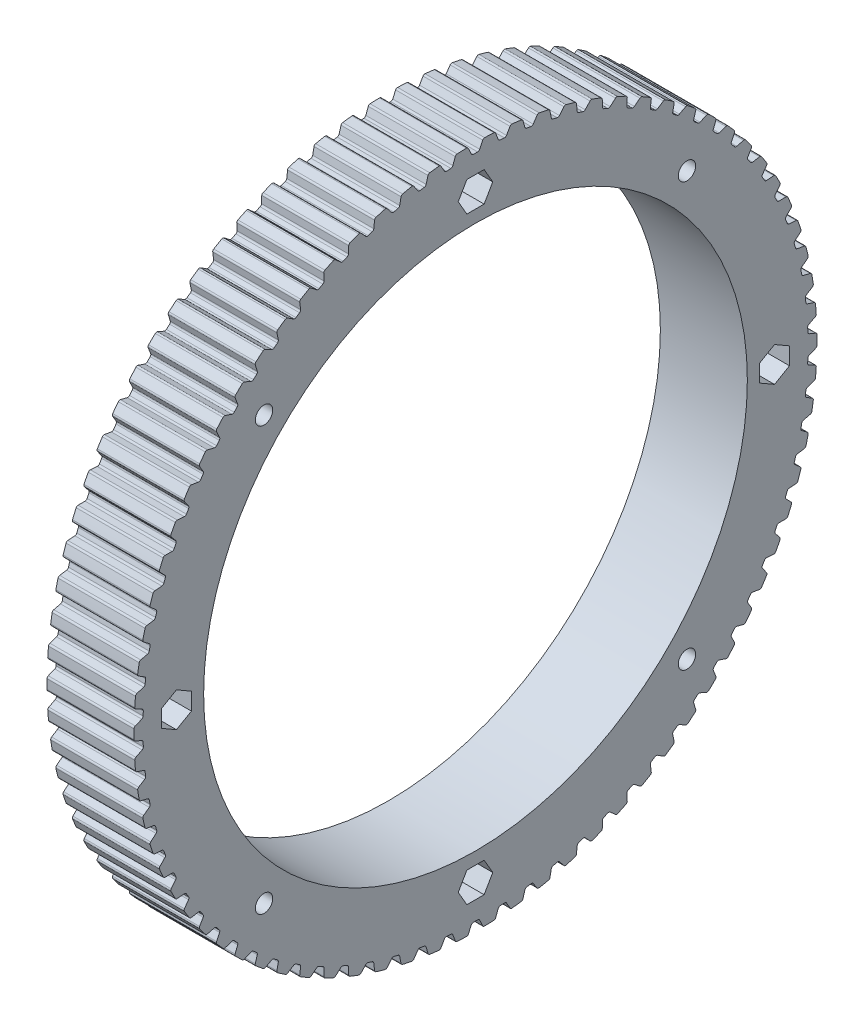
from build123d import *

# Parameters (mm, degrees)
CHAMFER_1_SIZE           = 1
SKETCH_4_W               = 8
SKETCH_4_H               = 3.299999952
CUT_EXTRUDE_1_DEPTH      = 91.633566861
CUT_EXTRUDE_2_REACH      = 92.634
PATTERN_CIRCULAR_3_COUNT = 78
CUT_EXTRUDE_4_DEPTH      = 91.242238534
CUT_EXTRUDE_4_DEPTH_BACK = 91.242238534
SKETCH_7_R               = 50
SKETCH_7_R_2             = 1.6
CUT_EXTRUDE_5_DEPTH      = 5
CUT_EXTRUDE_6_DEPTH      = 5


with BuildPart() as part:
    # 草图1 → 旋转1 (revolve)
    with BuildSketch(Plane.XY, mode=Mode.PRIVATE) as revolve_1_sk:
        Polygon((0, 11.5922), (0, 62.811), (16, 62.811), (16, 23.1844), (18, 23.1844), (18, 11.5922), align=None)
    revolve(revolve_1_sk.sketch.rotate(Axis((0, 0, 0), (1, 0, 0)), 90), axis=Axis((0, 0, 0), (1, 0, 0)))

    # 倒角1
    chamfer_1_edges = [part.edges().sort_by_distance(p)[0] for p in [
        (0, 0, -11.5922),
        (18, 0, -11.5922),
    ]]
    chamfer(chamfer_1_edges, length=CHAMFER_1_SIZE)

    # 草图4 → 切除-拉伸1 (cut, through all)
    with BuildSketch(Plane.ZY):
        with Locations((0, 12.530216005)):
            Rectangle(SKETCH_4_W, SKETCH_4_H)
    extrude(amount=-CUT_EXTRUDE_1_DEPTH, mode=Mode.SUBTRACT)

    # 草图6 → 切除-拉伸2 (cut, up to next)
    with BuildSketch(Plane(origin=(0, 0, 0), x_dir=(0, 0, -1), z_dir=(1, 0, 0)), mode=Mode.PRIVATE) as cut_extrude_2_sk1:
        with BuildLine():
            Line((1.318430055, 62.569446614), (0.771442548, 61.396428119))
            ThreePointArc((0.771442548, 61.396428119), (0.619025206, 61.223197616), (0.39719372, 61.159710252))
            ThreePointArc((0.39719372, 61.159710252), (0, 61.161), (-0.39719372, 61.159710252))
            ThreePointArc((-0.39719372, 61.159710252), (-0.619025206, 61.223197616), (-0.771442548, 61.396428119))
            Line((-0.771442548, 61.396428119), (-1.318430055, 62.569446614))
            ThreePointArc((-1.318430055, 62.569446614), (-1.462939702, 62.732031287), (-1.672948176, 62.788716864))
            ThreePointArc((-1.672948176, 62.788716864), (-1.862873117, 62.783369014), (-2.052781012, 62.777446676))
            Line((-2.052781012, 62.777446676), (-2.66825474, 64.097334344))
            ThreePointArc((-2.66825474, 64.097334344), (0, 64.152847586), (2.66825474, 64.097334344))
            Line((2.66825474, 64.097334344), (2.052781012, 62.777446676))
            ThreePointArc((2.052781012, 62.777446676), (1.862873117, 62.783369014), (1.672948176, 62.788716864))
            ThreePointArc((1.672948176, 62.788716864), (1.462939702, 62.732031287), (1.318430055, 62.569446614))
        make_face()
    cut_extrude_2_tool1 = extrude(cut_extrude_2_sk1.sketch, amount=CUT_EXTRUDE_2_REACH, mode=Mode.PRIVATE) & part.part
    cut_extrude_2 = cut_extrude_2_tool1.solids().sort_by_distance((0, 63.003061, 0))[0]
    add(cut_extrude_2, mode=Mode.SUBTRACT)

    # 阵列(圆周)3: 切除-拉伸2 ×78 about axis
    pattern_circular_3_axis = Axis((0, 0, 0), (1, 0, 0))
    for i in range(1, PATTERN_CIRCULAR_3_COUNT):
        add(cut_extrude_2.rotate(pattern_circular_3_axis, i * 360 / PATTERN_CIRCULAR_3_COUNT), mode=Mode.SUBTRACT)

    # 草图7 → 切除-拉伸4 (cut, two sides: drawn at the far end of the back side and taken through both)
    with BuildSketch(Plane(origin=(16, 0, 0), x_dir=(0, 0, -1), z_dir=(1, 0, 0)).offset(-CUT_EXTRUDE_4_DEPTH_BACK)):
        Circle(SKETCH_7_R)
        with Locations((0, 55)):
            Circle(SKETCH_7_R_2)
        with Locations((38.890872965, 38.890872965)):
            Circle(SKETCH_7_R_2)
        with Locations((55, 0)):
            Circle(SKETCH_7_R_2)
        with Locations((38.890872965, -38.890872965)):
            Circle(SKETCH_7_R_2)
        with Locations((0, -55)):
            Circle(SKETCH_7_R_2)
        with Locations((-38.890872965, -38.890872965)):
            Circle(SKETCH_7_R_2)
        with Locations((-55, 0)):
            Circle(SKETCH_7_R_2)
        with Locations((-38.890872965, 38.890872965)):
            Circle(SKETCH_7_R_2)
    extrude(amount=CUT_EXTRUDE_4_DEPTH + CUT_EXTRUDE_4_DEPTH_BACK, mode=Mode.SUBTRACT)

    # 草图9 → 切除-拉伸5 (cut)
    with BuildSketch(Plane(origin=(16, 0, 0), x_dir=(0, 0, -1), z_dir=(1, 0, 0))):
        Polygon((55, -3.175426481), (57.75, -1.58771324), (57.75, 1.58771324), (55, 3.175426481), (52.25, 1.58771324), (52.25, -1.58771324), align=None)
        Polygon((3.175426481, 55), (1.58771324, 57.75), (-1.58771324, 57.75), (-3.175426481, 55), (-1.58771324, 52.25), (1.58771324, 52.25), align=None)
        Polygon((-3.175426481, -55), (-1.58771324, -57.75), (1.58771324, -57.75), (3.175426481, -55), (1.58771324, -52.25), (-1.58771324, -52.25), align=None)
        Polygon((-55, 3.175426481), (-57.75, 1.58771324), (-57.75, -1.58771324), (-55, -3.175426481), (-52.25, -1.58771324), (-52.25, 1.58771324), align=None)
    extrude(amount=-CUT_EXTRUDE_5_DEPTH, mode=Mode.SUBTRACT)

    # 草图10 → 切除-拉伸6 (cut)
    with BuildSketch(Plane.ZY):
        Polygon((36.645507368, -41.136238563), (39.712733815, -41.958099412), (41.958099412, -39.712733815), (41.136238563, -36.645507368), (38.069012116, -35.823646518), (35.823646518, -38.069012116), align=None)
        Polygon((41.136238563, 36.645507368), (41.958099412, 39.712733815), (39.712733815, 41.958099412), (36.645507368, 41.136238563), (35.823646518, 38.069012116), (38.069012116, 35.823646518), align=None)
        Polygon((-41.136238563, -36.645507368), (-41.958099412, -39.712733815), (-39.712733815, -41.958099412), (-36.645507368, -41.136238563), (-35.823646518, -38.069012116), (-38.069012116, -35.823646518), align=None)
        Polygon((-36.645507368, 41.136238563), (-39.712733815, 41.958099412), (-41.958099412, 39.712733815), (-41.136238563, 36.645507368), (-38.069012116, 35.823646518), (-35.823646518, 38.069012116), align=None)
    extrude(amount=-CUT_EXTRUDE_6_DEPTH, mode=Mode.SUBTRACT)


solid = part.part
